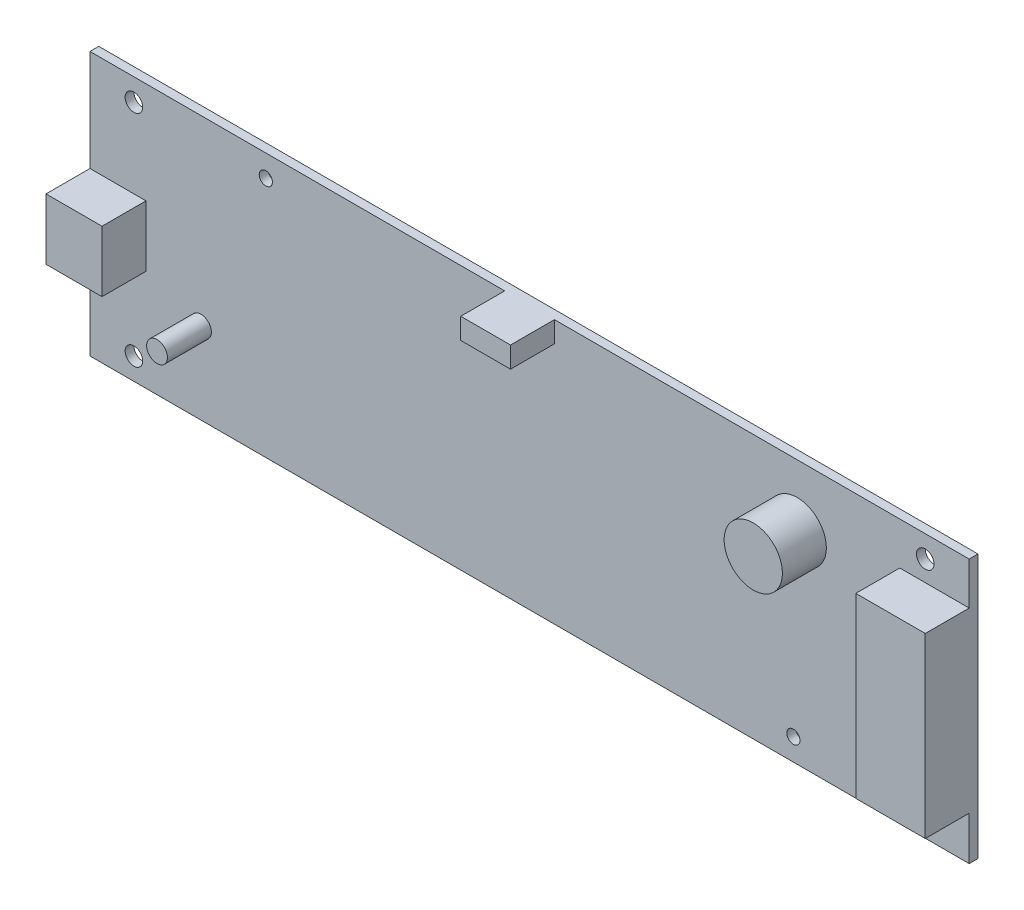
from build123d import *

# Parameters (mm, degrees)
SKETCH1_W           = 100
SKETCH1_H           = 30
SKETCH1_R           = 1
BOSS_EXTRUDE1_DEPTH = 1
SKETCH2_R           = 3.312148645
SKETCH2_R_2         = 1.182707094
SKETCH2_W           = 7.897065894
SKETCH2_H           = 20.201539664
SKETCH2_W_2         = 5.658967966
SKETCH2_H_2         = 2.382698796
SKETCH2_W_3         = 6.371052581
SKETCH2_H_3         = 6.939357654
BOSS_EXTRUDE2_DEPTH = 5
SKETCH3_W           = 5
SKETCH3_H           = 5
BOSS_EXTRUDE3_DEPTH = 1
SKETCH4_R           = 1
BOSS_EXTRUDE4_DEPTH = 1
SKETCH5_R           = 0.75
CUT_EXTRUDE1_DEPTH  = 10


with BuildPart() as part:
    # Sketch1 → Boss-Extrude1 (new body)
    with BuildSketch(Plane.XY):
        Rectangle(SKETCH1_W, SKETCH1_H)
        with Locations((-45, -12.5)):
            Circle(SKETCH1_R, mode=Mode.SUBTRACT)
        with Locations((-45, 12.5)):
            Circle(SKETCH1_R, mode=Mode.SUBTRACT)
        with Locations((45, 12.5)):
            Circle(SKETCH1_R, mode=Mode.SUBTRACT)
        with Locations((45, -12.5)):
            Circle(SKETCH1_R, mode=Mode.SUBTRACT)
    extrude(amount=BOSS_EXTRUDE1_DEPTH)

    # Sketch2 → Boss-Extrude2 (add)
    with BuildSketch(Plane.XY.offset(1)):
        with Locations((30.440398969, 7.974336126)):
            Circle(SKETCH2_R)
        with Locations((-37.372165455, -5.749563916)):
            Circle(SKETCH2_R_2)
        with Locations((46.051467053, 0.07257894)):
            Rectangle(SKETCH2_W, SKETCH2_H)
        with Locations((0, 13.808650602)):
            Rectangle(SKETCH2_W_2, SKETCH2_H_2)
        with Locations((-46.814473709, 0)):
            Rectangle(SKETCH2_W_3, SKETCH2_H_3)
    extrude(amount=BOSS_EXTRUDE2_DEPTH)

    # Sketch3 → Boss-Extrude3 (add)
    with BuildSketch(Plane(origin=(0, 0, 0), x_dir=(-1, 0, 0), z_dir=(0, 0, -1))):
        with Locations((-12.5, -7)):
            Rectangle(SKETCH3_W, SKETCH3_H)
        with Locations((-37.5, -7)):
            Rectangle(SKETCH3_W, SKETCH3_H)
        with Locations((37.5, -7)):
            Rectangle(SKETCH3_W, SKETCH3_H)
        with Locations((12.5, -7)):
            Rectangle(SKETCH3_W, SKETCH3_H)
    extrude(amount=BOSS_EXTRUDE3_DEPTH)

    # Sketch4 → Boss-Extrude4 (add)
    with BuildSketch(Plane(origin=(0, 0, -1), x_dir=(-1, 0, 0), z_dir=(0, 0, -1))):
        with Locations((-37.5, -7)):
            Circle(SKETCH4_R)
        with Locations((-12.5, -7)):
            Circle(SKETCH4_R)
        with Locations((12.5, -7)):
            Circle(SKETCH4_R)
        with Locations((37.5, -7)):
            Circle(SKETCH4_R)
    extrude(amount=BOSS_EXTRUDE4_DEPTH)

    # Sketch5 → Cut-Extrude1 (cut)
    with BuildSketch(Plane.XY.offset(1)):
        with Locations((30, -12.5)):
            Circle(SKETCH5_R)
        with Locations((-30, 12.5)):
            Circle(SKETCH5_R)
    extrude(amount=-CUT_EXTRUDE1_DEPTH, mode=Mode.SUBTRACT)


solid = part.part
